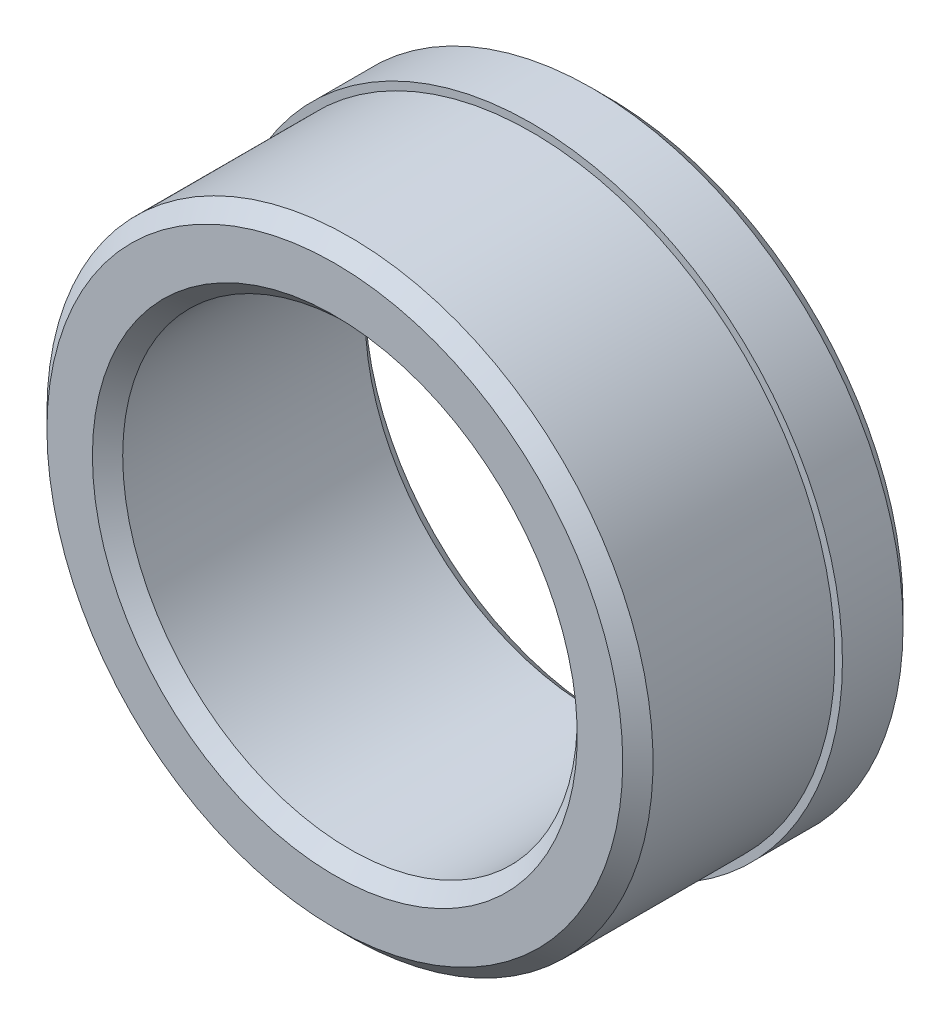
SolidWorks part; units mm, degrees
material "20 steel"
ref_plane "Front Plane" through (0, 0, 0) normal (0, 0, 1) x (1, 0, 0)
ref_plane "Top Plane" through (0, 0, 0) normal (0, 1, 0) x (1, 0, 0)
ref_plane "Right Plane" through (0, 0, 0) normal (1, 0, 0) x (0, 0, -1)
other "Configuration Table"
sketch "Sketch1" plane through (0, 0, 0) normal (1, 0, 0) x (0, 0, -1)
  line L1 (0, 0) -> (-36, 0)
  line L2 (0, 0) -> (0, 40)
  line L3 (0, 40) -> (-36, 40)
  line L4 (-36, 0) -> (-36, 40)
  line L5 (0, 0) -> (-36, 0)
  line L6 (0, 0) -> (0, 30)
  line L7 (0, 30) -> (-36, 30)
  line L8 (-36, 0) -> (-36, 30)
  line L9 (0, 0) -> (-10, 0)
  line L10 (0, 0) -> (0, 41)
  line L11 (0, 41) -> (-10, 41)
  line L12 (-10, 0) -> (-10, 41)
  dimension "D1" = 36
  dimension "D2" = 40
  dimension "D3" = 41
  dimension "D4" = 30
  dimension "D5" = 10
revolve "Revolve1" add sketch "Sketch1" angle 360 about L1
chamfer "Chamfer1" distance 2 angle 45 4 edges at (-30, 0, 0) (-41, 0, 0) (-30, 0, 36) (-40, 0, 36)
